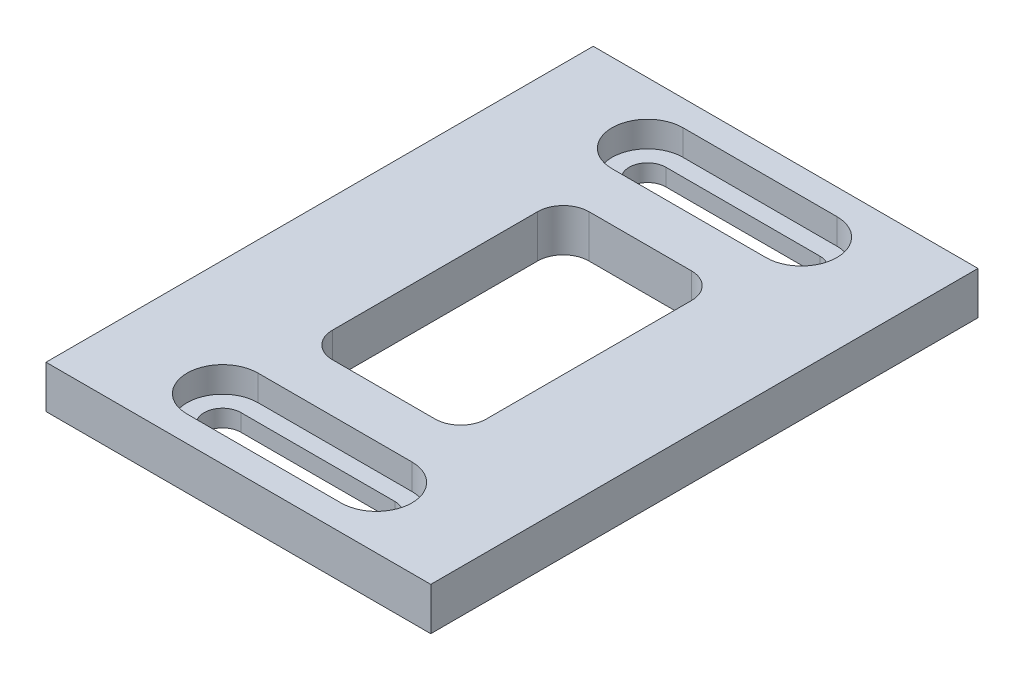
from build123d import *

# Parameters (mm, degrees)
SKETCH1_W           = 45
SKETCH1_H           = 64
BOSS_EXTRUDE1_DEPTH = 5
SKETCH_2_3_W        = 18
SKETCH_2_3_H        = 30
CUT_EXTRUDE1_DEPTH  = 40.436658073
CUT_EXTRUDE2_DEPTH  = 3
FILLET1_R           = 3


with BuildPart() as part:
    # Sketch1 → Boss-Extrude1 (new body)
    with BuildSketch(Plane(origin=(0, 0, 0), x_dir=(1, 0, 0), z_dir=(0, 1, 0))):
        Rectangle(SKETCH1_W, SKETCH1_H)
    extrude(amount=BOSS_EXTRUDE1_DEPTH)

    # Sketch 2_3 → Cut-Extrude1 (cut, through all)
    with BuildSketch(Plane(origin=(0, 5, 0), x_dir=(1, 0, 0), z_dir=(0, 1, 0))):
        Rectangle(SKETCH_2_3_W, SKETCH_2_3_H)
        with BuildLine():
            Line((-9, -22.7), (9, -22.7))
            ThreePointArc((9, -22.7), (11.15, -24.85), (9, -27))
            Line((9, -27), (-9, -27))
            ThreePointArc((-9, -27), (-11.15, -24.85), (-9, -22.7))
        make_face()
        with BuildLine():
            Line((-9, 22.7), (9, 22.7))
            ThreePointArc((9, 22.7), (11.15, 24.85), (9, 27))
            Line((9, 27), (-9, 27))
            ThreePointArc((-9, 27), (-11.15, 24.85), (-9, 22.7))
        make_face()
    extrude(amount=-CUT_EXTRUDE1_DEPTH, mode=Mode.SUBTRACT)

    # Sketch 2_3 2 → Cut-Extrude2 (cut)
    with BuildSketch(Plane(origin=(0, 5, 0), x_dir=(1, 0, 0), z_dir=(0, 1, 0))):
        with BuildLine():
            Line((-9, -20.7), (9, -20.7))
            ThreePointArc((9, -20.7), (13.15, -24.85), (9, -29))
            Line((9, -29), (-9, -29))
            ThreePointArc((-9, -29), (-13.15, -24.85), (-9, -20.7))
        make_face()
        with BuildLine():
            Line((-9, 20.7), (9, 20.7))
            ThreePointArc((9, 20.7), (13.15, 24.85), (9, 29))
            Line((9, 29), (-9, 29))
            ThreePointArc((-9, 29), (-13.15, 24.85), (-9, 20.7))
        make_face()
    extrude(amount=-CUT_EXTRUDE2_DEPTH, mode=Mode.SUBTRACT)

    # Fillet1
    fillet1_edges = [part.edges().sort_by_distance(p)[0] for p in [
        (-9, 2.5, -15),
        (9, 2.5, -15),
        (9, 2.5, 15),
        (-9, 2.5, 15),
    ]]
    fillet(fillet1_edges, radius=FILLET1_R)


solid = part.part
